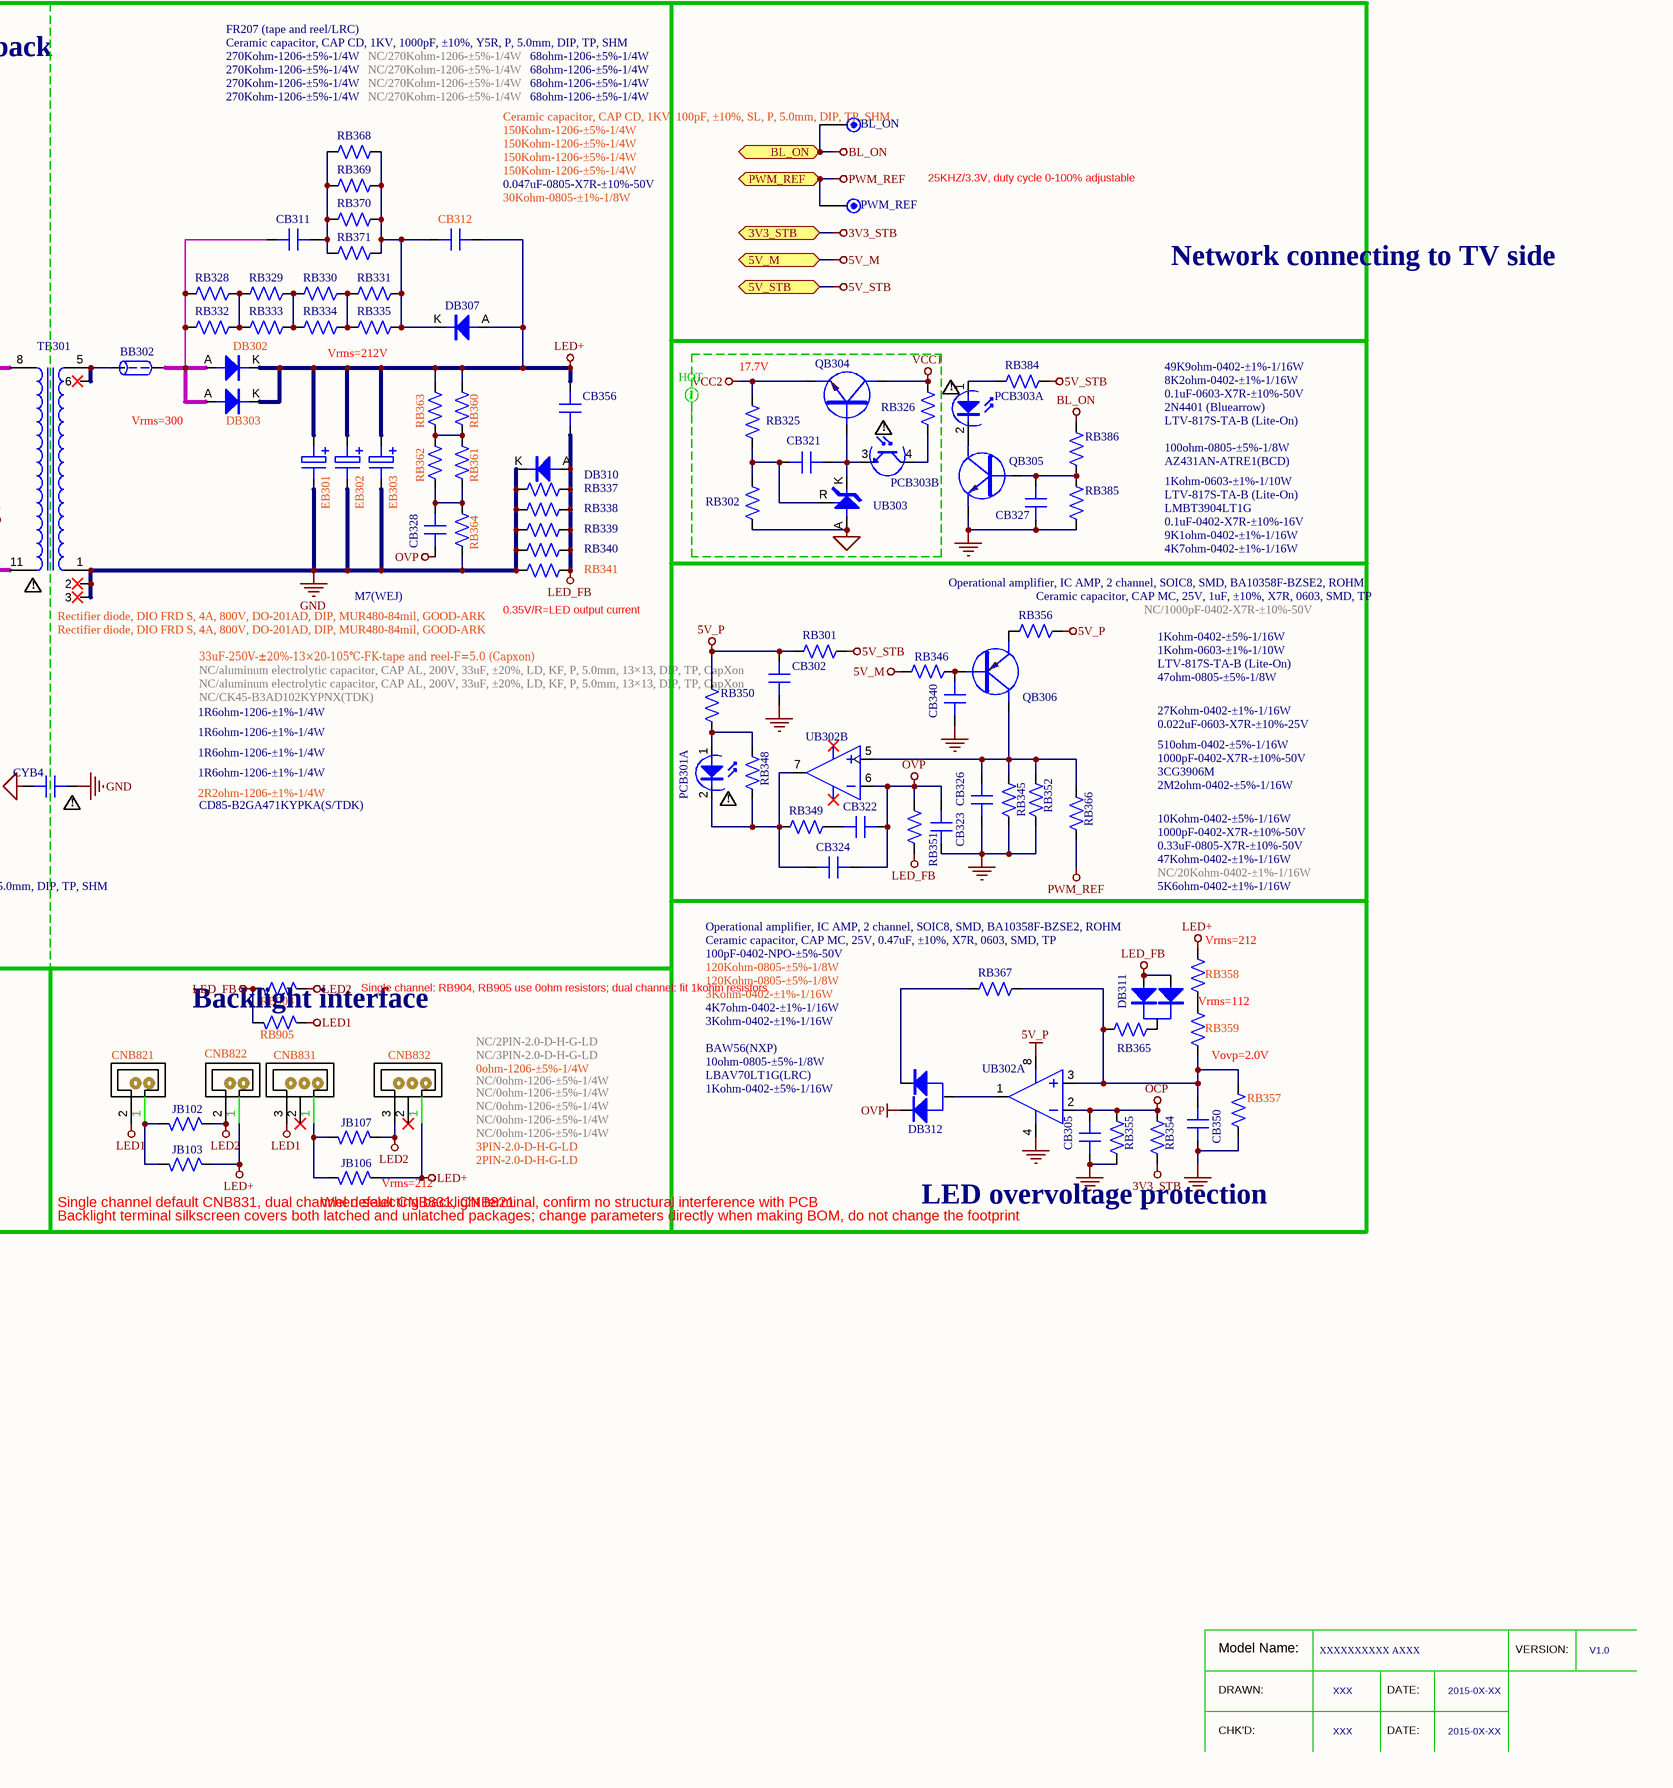
[diagram p0: PCBE84277.SchDoc, bottom right]
# Altium project MISC84277-14.PrjPCB (part 5 of 10)

## Sheet PCBE84277.SchDoc: MISC84277 (continued)

### Parts
BB101  φ3.5×6.0×0.65mm-CP (tape and reel/Xiuyida)  [LB/3.5*6*15]
BB201  φ3.5×6.0×0.65mm-CP (tape and reel/Xiuyida)  [LB/3.5*6*12.5]
BB301  φ3.5×6.0×0.65mm-CP (tape and reel/Xiuyida)  [LB/3.5*6*12.5]
BB302  φ3.5×6.0×0.65mm-CP (tape and reel/Xiuyida)  [LB/3.5*6*12.5]
BL_ON  TEST  [TP_BL]  (value not drawn)
CB2  B32672P4474K006(EPCOS)  [CAP18*7-V-15]
CB3  B32672P4474K006(EPCOS)  [CAP18*7-V-15]
CB101  100pF-0402-NPO-±5%-50V  [C0402]
CB102  0.1uF-0603-X7R-±10%-50V  [C0603]
CB103  1000pF-0402-X7R-±10%-50V  [C0402]
CB109  0.1uF-0603-X7R-±10%-50V  [C0603]
CB110  NC/1000pF-0402-X7R-±10%-50V  [C0402]
CB111  NC/1uF-0805-X7R-±10%-25V  [C0805]
CB112  NC/1uF-0805-X7R-±10%-25V  [C0805]
CB113  220PF-0805-NPO-±10%-200V  [C0805]
CB114  C242G472J20A201 (tape and reel/Faraday)  [CAP8*2.5-V-5]
CB116  Ceramic capacitor, CAP CD, 1KV, 100pF, ±10%, SL, P, 5.0mm, DIP, TP, SHM  [CAP7.5*2.5-V-5]
CB118  1000pF-0805-NPO-±10%-200V  [C0805]
CB201  0.047uF-0603-X7R-±10%-25V  [C0603]
CB204  NC/ceramic capacitor, CAP CD, 1KV, 4700pF, ±20%, Y5U, P, 5.0mm, DIP, TP, TongHao  [CAP9.8*4-V-5]
CB205  220pF-0402-NPO-±5%-50V  [C0402]
CB206  0.1uF-0603-X7R-±10%-50V  [C0603]
CB209  Ceramic capacitor, CAP CD, 1KV, 100pF, ±10%, SL, P, 5.0mm, DIP, TP, SHM  [CAP7.5*2.5-V-5]
CB211  CC45SL3AD470JYPNA(TDK)  [CAP7.5*2.5-V-5]
CB212  0.22uF-0805-X7R-±10%-50V  [C0805]
CB221  4700pF-0402-X7R-±10%-50V  [C0402]
CB301  4700pF-0402-X7R-±10%-50V  [C0402]
CB302  Ceramic capacitor, CAP MC, 25V, 1uF, ±10%, X7R, 0603, SMD, TP  [C0603]
CB303  100pF-0402-NPO-±5%-50V  [C0402]
CB304  0.1uF-0603-X7R-±10%-50V  [C0603]
CB305  100pF-0402-NPO-±5%-50V  [C0402]
CB306  C242G472J20A201 (tape and reel/Faraday)  [CAP8*2.5-V-5]
CB311  Ceramic capacitor, CAP CD, 1KV, 1000pF, ±10%, Y5R, P, 5.0mm, DIP, TP, SHM  [CAP7.5*2.5-V-5]
CB312  Ceramic capacitor, CAP CD, 1KV, 100pF, ±10%, SL, P, 5.0mm, DIP, TP, SHM  [CAP7.5*2.5-V-5]
CB316  Ceramic capacitor, CAP CD, 1KV, 100pF, ±10%, SL, P, 5.0mm, DIP, TP, SHM  [CAP7.5*2.5-V-5]
CB321  0.1uF-0603-X7R-±10%-50V  [C0603]
CB322  0.022uF-0603-X7R-±10%-25V  [C0603]
CB323  1000pF-0402-X7R-±10%-50V  [C0402]
CB324  NC/1000pF-0402-X7R-±10%-50V  [C0402]
CB326  0.33uF-0805-X7R-±10%-50V  [C0805]
CB327  0.1uF-0402-X7R-±10%-16V  [C0402]
CB328  0.047uF-0805-X7R-±10%-50V  [C0805]
CB340  1000pF-0402-X7R-±10%-50V  [C0402]
CB350  Ceramic capacitor, CAP MC, 25V, 0.47uF, ±10%, X7R, 0603, SMD, TP  [C0603]
CB356  NC/CK45-B3AD102KYPNX(TDK)  [CAP8.5*4-V-5]
CB951  NC/0.1uF-0402-X7R-±10%-16V  [C0402]
CNB1  Connect jack, 2Pin, D7.92, L, SNAP, Fool-proofing, nature, L=2.8mm, DIP, AMA  [CON2-H7.92]
CNB2  2PIN-2.0-D-H-G-LD  [SIP2/2.0D-1]
CNB812  NC/2×4PIN-2.0-L-H-F-gold plated-LK  [SIP2*4H/2.0DF-1]
CNB821  NC/2PIN-2.0-D-H-G-LD  [SIP2/2.0D-CP]
CNB822  2PIN-2.0-D-H-G-LD  [SIP2/2.0D-CP]
CNB831  NC/3PIN-2.0-D-H-G-LD  [SIP3/2.0D-CP]
CNB832  3PIN-2.0-D-H-G-LD  [SIP3/2.0D-CP]
CXB1  X capacitor, CAP X2, MP, 275VAC, 0.47uF, ±10%, S, 15mm-Mini, PC, DIP, BM  [CAP18*8.5-V-15]
CYB1  CD70-B2GA221KYPKA(S/TDK)  [CAP13*4.5-V-10]
CYB2  CD70-B2GA221KYPKA(S/TDK)  [CAP13*4.5-V-10]
CYB3  CD85-B2GA471KYPKA(S/TDK)  [CAP13*4.5-V-10]
CYB4  CD85-B2GA471KYPKA(S/TDK)  [CAP13*4.5-V-10]
DB1  1N5408G (tape and reel / GOOD-ARK)  [D3-H-20]
DB2  1N5408G (tape and reel / GOOD-ARK)  [D3-H-20]
DB3  1N5408G (tape and reel / GOOD-ARK)  [D3-H-20]
DB4  1N5408G (tape and reel / GOOD-ARK)  [D3-H-20]
DB101  MBRB10150CT(GOOD-ARK)  [D2PAK3]
DB102  LBAV70LT1G(LRC)  [SO-23]
DB105  FR107 (tape and reel/LRC)  [D1-H-12.5]
DB106  FR207 (tape and reel/LRC)  [D2-H-17.5]
DB201  Rectifier diode, DIO FRD S, 8A, 600V, ITO-220AC, DIP, UGF8J C0G, TSC  [TO-220-AK-H]
DB202  NC/GS3J-B(GULF)  [DIODE-SMB-1]
DB203  NC/GS3J-B(GULF)  [DIODE-SMB-1]
DB204  LBAV70LT1G(LRC)  [SO-23]
DB302  Rectifier diode, DIO FRD S, 4A, 800V, DO-201AD, DIP, MUR480-84mil, GOOD-ARK  [D3-H-20]
DB303  Rectifier diode, DIO FRD S, 4A, 800V, DO-201AD, DIP, MUR480-84mil, GOOD-ARK  [D3-H-20]
DB306  FR207 (tape and reel/LRC)  [D2-H-17.5]
DB307  FR207 (tape and reel/LRC)  [D2-H-17.5]
DB310  M7(WEJ)  [DIODE-S-2]
DB311  LBAV70LT1G(LRC)  [SO-23]
DB312  BAW56(NXP)  [SO-23-1]
DB370  NC/FF7  [DIODE-S-14]
DB371  NC/FF7  [DIODE-S-14]
DB901  NC/LBAV70LT1G(LRC)  [SO-23]
DB951  NC/LBAV70LT1G(LRC)  [SO-23]
EB101  470uF-25V-±20%-10×12.5-105℃-GF-tape and reel-F=5.0 (CapXon)  [EC(10*12.5)-V-5]
EB102  NC/270uF-16V-±20%-8×11.5-105℃-PS-short leads-F=3.5 (Capxon)  [EC(8*11)-V-3.5]
EB103  470uF-25V-±20%-10×12.5-105℃-GF-tape and reel-F=5.0 (CapXon)  [EC(10*12.5)-V-5]
EB106  47uF-50V-±20%-6.3×11-105℃-GH-tape and reel-F=2.5 (CapXon)  [EC(6.3*11)-V-2.5]
EB107  10uF-50V-±20%-5×11-105℃-GH-tape and reel-F=2.5 (CapXon)  [EC(5*11)-V-2.5]
EB201  100uF-450V-±20%-16×35.5-105℃-KM-bent leads (H=8.1mm) (Capxon)  [EC(16*37)-H-7.5]
EB301  33uF-250V-±20%-13×20-105℃-FK-tape and reel-F=5.0 (Capxon)  [EC(13*20)-H-5]
EB302  NC/aluminum electrolytic capacitor, CAP AL, 200V, 33uF, ±20%, LD, KF, P, 5.0mm, 13×13, DIP, TP, CapXon  [EC(13*13)-V-5]
EB303  NC/aluminum electrolytic capacitor, CAP AL, 200V, 33uF, ±20%, LD, KF, P, 5.0mm, 13×13, DIP, TP, CapXon  [EC(13*13)-V-5]
EVA1  NC/7×7×3mm-C-4305 fireproof foam-black  [EVA(7*7*3)]
EVA2  NC/7×7×3mm-C-4305 fireproof foam-black  [EVA(7*7*3)]
EVA3  NC/7×7×3mm-C-4305 fireproof foam-black  [EVA(7*7*3)]
EVA4  NC/7×7×3mm-C-4305 fireproof foam-black  [EVA(7*7*3)]
EVA5  NC/7×7×3mm-C-4305 fireproof foam-black  [EVA(7*7*3)]
EVA6  NC/7×7×3mm-C-4305 fireproof foam-black  [EVA(7*7*3)]
EVA7  NC/7×7×3mm-C-4305 fireproof foam-black  [EVA(7*7*3)]
FB1  2010T3.15A250VA1 (tape and reel/Huade)  [FUSE8.5*4-V-5]
GD1  7.00×8.35mm-nylon-white-WQM  [Fixed]
GD2  7.00×8.35mm-nylon-white-WQM  [Fixed]
GD3  7.00×8.35mm-nylon-white-WQM  [Fixed]
GD4  7.00×8.35mm-nylon-white-WQM  [Fixed]
GL1  SLD-8854W  [Silica gel-20]
GL2  SLD-8854W  [Silica gel-10]
GL3  NC/SLD-8854W  [Silica gel-10]
GL4  SLD-8854W  [Silica gel-10]
HSB2  40×25×5.0-black-with pins (thickness=1.5mm)-FR  [HS018]
HSB3  50×25×5.0-black-with pins (thickness=1.5mm)-FR  [HS033]
HSB6  NC/17.5×14.5×0.5- natural finish -Cu-MRD  [HS038]
JB102  NC/0ohm-1206-±5%-1/4W  [R1206]
JB103  NC/0ohm-1206-±5%-1/4W  [R1206]
JB106  NC/0ohm-1206-±5%-1/4W  [R1206]
JB107  NC/0ohm-1206-±5%-1/4W  [R1206]
LB1  SYDR1212-L003-EDL  [L/LC2/15*14.5-V7.5]
LB202  SYEQ2612-L250uA-SQ  [T/EQ2512*11]
LCB1  SYT10-L002-EDL  [L/LC4/13.5*10-V-7*6]
LCB2  SYT14-L003-JM  [L/LC4/T14-H-8*6]
MB1  PM3.0×8.0×5.5mm-silver-double washer  [SCREW]
MB2  PM3.0×8.0×5.5mm-silver-double washer  [SCREW]
ML1  Mylar sheet, Mylar, XXX  [Mylar]
MOVB1  TVR10561KSC3AGGW (short leads/Weiqin)  [VR(13*5)-V-7.5]
NTCB2  SCK102R55AMBY502 (short leads/Weiqin)  [NTC(10*5)-V5]
PCB101  LTV-817S-TA-B (Lite-On)  [OC4-S-1]  (parts A,B of 2)
PCB301  LTV-817S-TA-B (Lite-On)  [OC4-S-1]  (parts A,B of 2)
PCB303  LTV-817S-TA-B (Lite-On)  [OC4-S-1]  (parts A,B of 2)
PWM_REF  TEST  [TP_BL]  (value not drawn)
QB101  MOSFET, NMOS, 5A, 700V, 0.9ohm@ID=2.5A@VGS=10V, TO-252, MMD70R900PRH, MAGNACHIP  [TO-252-GDS]
QB102  3CG3906M  [SOT-23]
QB201  MDF13N50BTH(Magnachip)  [TO-220-GDS-H]
QB201和散热片之间  0.05g  [PCB_TIME]
QB301  MDF7N65BTH(Magnachip)  [TO-220-GDS-H]
QB301和散热片之间  0.05g  [PCB_TIME]
QB302  3CG3906M  [SOT-23]
QB304  2N4401 (Bluearrow)  [TO-92-EBC]
QB305  LMBT3904LT1G  [SOT-23]
QB306  3CG3906M  [SOT-23]
QB911  NC/2SD1857L-Q-T9N-B(UTC)  [TO-92-ECB]
QB921  NC/2SD1857L-Q-T9N-B(UTC)  [TO-92-ECB]
QB931  NC/2SD1857L-Q-T9N-B(UTC)  [TO-92-ECB]
QB941  NC/2SD1857L-Q-T9N-B(UTC)  [TO-92-ECB]
QB951  NC/LMBT3904LT1G  [SOT-23]
RB1  1M2ohm-1206-±5%-1/4W  [R1206]
RB2  1M2ohm-1206-±5%-1/4W  [R1206]
RB3  1M2ohm-1206-±5%-1/4W  [R1206]
RB4  1M2ohm-1206-±5%-1/4W  [R1206]
RB101  330Kohm-1206-±5%-1/4W  [R1206]
RB102  330Kohm-1206-±5%-1/4W  [R1206]
RB103  10Kohm-0402-±1%-1/16W  [R0402]
RB104  47Kohm-0402-±1%-1/16W  [R0402]
RB105  510ohm-0402-±5%-1/16W  [R0402]
RB106  68ohm-0805-±5%-1/8W  [R0805]
RB107  510ohm-0402-±5%-1/16W  [R0402]
RB108  20ohm-0805-±5%-1/8W  [R0805]
RB109  10Kohm-0402-±5%-1/16W  [R0402]
RB110  10ohm-1206-±5%-1/4W  [R1206]
RB114  10ohm-1206-±5%-1/4W  [R1206]
RB115  10ohm-1206-±5%-1/4W  [R1206]
RB116  10ohm-1206-±5%-1/4W  [R1206]
RB117  10ohm-1206-±5%-1/4W  [R1206]
RB118  10ohm-1206-±5%-1/4W  [R1206]
RB123  47ohm-1206-±5%-1/4W  [R1206]
RB124  47ohm-1206-±5%-1/4W  [R1206]
RB131  2Kohm-0603-±5%-1/10W  [R0603]
RB132  3Kohm-0402-±1%-1/16W  [R0402]
RB133  3Kohm-0402-±1%-1/16W  [R0402]
RB134  4K7ohm-0402-±1%-1/16W  [R0402]
RB135  18Kohm-0402-±1%-1/16W  [R0402]
RB141  NC/2Mohm-1206-±5%-1/4W  [R1206]
RB142  NC/2Mohm-1206-±5%-1/4W  [R1206]
RB143  NC/0ohm-0402-±5%-1/16W  [R0402]
RB144  100Kohm-1206-±5%-1/4W  [R1206]
RB145  100Kohm-1206-±5%-1/4W  [R1206]
RB146  100Kohm-1206-±5%-1/4W  [R1206]
RB147  100Kohm-1206-±5%-1/4W  [R1206]
RB148  MOF-0R27ohm-±5%-2WS (tape and reel/Futaba)  [R2-H-17.5]
RB201  1Mohm-1206-±1%-1/4W  [R1206]
RB202  1Mohm-1206-±1%-1/4W  [R1206]
RB203  1Mohm-1206-±1%-1/4W  [R1206]
RB204  1Mohm-1206-±1%-1/4W  [R1206]
RB205  560kohm-0402-±1%-1/16W  [R0402]
RB206  27Kohm-0402-±1%-1/16W  [R0402]
RB209  39Kohm-0805-±1%-1/8W  [R0805]
RB210  10ohm-1206-±5%-1/4W  [R1206]
RB212  47ohm-0805-±5%-1/8W  [R0805]
RB213  20ohm-0805-±5%-1/8W  [R0805]
RB214  10Kohm-0402-±5%-1/16W  [R0402]
RB215  510ohm-0402-±5%-1/16W  [R0402]
RB217  MOF-0R1ohm-±5%-2WS (tape and reel/Futaba)  [R2-H-17.5]
RB218  1R6ohm-1206-±1%-1/4W  [R1206]
RB219  22ohm-1206-±5%-1/4W  [R1206]
RB220  22ohm-1206-±5%-1/4W  [R1206]
RB221  1Kohm-0402-±5%-1/16W  [R0402]
RB223  22ohm-1206-±5%-1/4W  [R1206]
RB224  22ohm-1206-±5%-1/4W  [R1206]
RB225  10Kohm-0402-±5%-1/16W  [R0402]
RB226  47Kohm-0402-±1%-1/16W  [R0402]
RB227  NC/0ohm-0402-±5%-1/16W  [R0402]
RB301  47ohm-0805-±5%-1/8W  [R0805]
RB302  8K2ohm-0402-±1%-1/16W  [R0402]
RB303  NC/10Kohm-0402-±5%-1/16W  [R0402]
RB304  47Kohm-0402-±1%-1/16W  [R0402]
RB305  510ohm-0402-±5%-1/16W  [R0402]
RB306  47ohm-0805-±5%-1/8W  [R0805]
RB307  510ohm-0402-±5%-1/16W  [R0402]
RB308  20ohm-0805-±5%-1/8W  [R0805]
RB309  10Kohm-0402-±5%-1/16W  [R0402]
RB310  MOF-0R22ohm-±5%-2WS (tape and reel/Futaba)  [R2-H-17.5]
RB314  10ohm-1206-±5%-1/4W  [R1206]
RB315  10ohm-1206-±5%-1/4W  [R1206]
RB317  330Kohm-1206-±5%-1/4W  [R1206]
RB318  330Kohm-1206-±5%-1/4W  [R1206]
RB319  330Kohm-1206-±5%-1/4W  [R1206]
RB320  330Kohm-1206-±5%-1/4W  [R1206]
RB321  330Kohm-1206-±5%-1/4W  [R1206]
RB322  330Kohm-1206-±5%-1/4W  [R1206]
RB323  330Kohm-1206-±5%-1/4W  [R1206]
RB324  330Kohm-1206-±5%-1/4W  [R1206]
RB325  49K9ohm-0402-±1%-1/16W  [R0402]
RB326  100ohm-0805-±5%-1/8W  [R0805]
RB328  270Kohm-1206-±5%-1/4W  [R1206]
RB329  270Kohm-1206-±5%-1/4W  [R1206]
RB330  270Kohm-1206-±5%-1/4W  [R1206]
RB331  270Kohm-1206-±5%-1/4W  [R1206]
RB332  NC/270Kohm-1206-±5%-1/4W  [R1206]
RB333  NC/270Kohm-1206-±5%-1/4W  [R1206]
RB334  NC/270Kohm-1206-±5%-1/4W  [R1206]
RB335  NC/270Kohm-1206-±5%-1/4W  [R1206]
RB337  1R6ohm-1206-±1%-1/4W  [R1206]
RB338  1R6ohm-1206-±1%-1/4W  [R1206]
RB339  1R6ohm-1206-±1%-1/4W  [R1206]
RB340  1R6ohm-1206-±1%-1/4W  [R1206]
RB341  2R2ohm-1206-±1%-1/4W  [R1206]
RB345  5K6ohm-0402-±1%-1/16W  [R0402]
RB346  510ohm-0402-±5%-1/16W  [R0402]
RB347  NC/MOF-300Kohm-±5%-2WS (tape and reel/Futaba)  [R2-H-17.5]
RB348  1Kohm-0402-±5%-1/16W  [R0402]
RB349  27Kohm-0402-±1%-1/16W  [R0402]
RB350  1Kohm-0603-±1%-1/10W  [R0603]
RB351  10Kohm-0402-±5%-1/16W  [R0402]
RB352  NC/20Kohm-0402-±1%-1/16W  [R0402]
RB354  3Kohm-0402-±1%-1/16W  [R0402]
RB355  4K7ohm-0402-±1%-1/16W  [R0402]
RB356  2M2ohm-0402-±5%-1/16W  [R0402]
RB357  3Kohm-0402-±1%-1/16W  [R0402]
RB358  120Kohm-0805-±5%-1/8W  [R0805]
RB359  120Kohm-0805-±5%-1/8W  [R0805]
RB360  150Kohm-1206-±5%-1/4W  [R1206]
RB361  150Kohm-1206-±5%-1/4W  [R1206]
RB362  150Kohm-1206-±5%-1/4W  [R1206]
RB363  150Kohm-1206-±5%-1/4W  [R1206]
RB364  30Kohm-0805-±1%-1/8W  [R0805]
RB365  10ohm-0805-±5%-1/8W  [R0805]
RB366  47Kohm-0402-±1%-1/16W  [R0402]
RB367  1Kohm-0402-±5%-1/16W  [R0402]
RB368  68ohm-1206-±5%-1/4W  [R1206]
RB369  68ohm-1206-±5%-1/4W  [R1206]
RB370  68ohm-1206-±5%-1/4W  [R1206]
RB371  68ohm-1206-±5%-1/4W  [R1206]
RB384  1Kohm-0603-±1%-1/10W  [R0603]
RB385  4K7ohm-0402-±1%-1/16W  [R0402]
RB386  9K1ohm-0402-±1%-1/16W  [R0402]
RB391  22ohm-1206-±5%-1/4W  [R1206]
RB392  22ohm-1206-±5%-1/4W  [R1206]
RB901  NC/470ohm-1206-±5%-1/4W  [R1206]
RB902  NC/470ohm-1206-±5%-1/4W  [R1206]
RB903  NC/470ohm-1206-±5%-1/4W  [R1206]
RB904  0ohm-1206-±5%-1/4W  [R1206]
RB905  NC/0ohm-1206-±5%-1/4W  [R1206]
RB911  NC/10ohm-1206-±5%-1/4W  [R1206]
RB912  NC/10ohm-1206-±5%-1/4W  [R1206]
RB913  NC/10ohm-1206-±5%-1/4W  [R1206]
RB921  NC/10ohm-1206-±5%-1/4W  [R1206]
RB922  NC/10ohm-1206-±5%-1/4W  [R1206]
RB923  NC/10ohm-1206-±5%-1/4W  [R1206]
RB931  NC/10ohm-1206-±5%-1/4W  [R1206]
RB932  NC/10ohm-1206-±5%-1/4W  [R1206]
RB933  NC/10ohm-1206-±5%-1/4W  [R1206]
RB941  NC/10ohm-1206-±5%-1/4W  [R1206]
RB942  NC/10ohm-1206-±5%-1/4W  [R1206]
RB943  NC/10ohm-1206-±5%-1/4W  [R1206]
RB951  NC/2Kohm-0402-±1%-1/16W  [R0402]
RB952  NC/20Kohm-1206-±5%-1/4W  [R1206]
TB101  SYEQ2612-T012A-YX  [T/EQ2512*11]
TB301  SYEQ32 (large-size constant current)  [T/EQ3214*11]
TP-TDT  (no value)  [TP-TDT]
UB101  PWM controller, IC PWM Controller, 65KHZ, SOT23-6, SMD, OB2273C, ON-Bright  [SOT-26]
UB102  AZ431AN-ATRE1(BCD)  [SOT-23-RAK]
UB201  PWM controller, IC PWM Controller, 300KHz, SOP-8, SMD, FAN7930CMX_G, Fairchild  [SO-8A]
UB301  PWM controller, IC PWM Controller, 65KHZ, SOT23-6, SMD, OB2273C, ON-Bright  [SOT-26]
UB302  Operational amplifier, IC AMP, 2 channel, SOIC8, SMD, BA10358F-BZSE2, ROHM  [SO-8A]  (parts A,B of 2)
UB303  AZ431AN-ATRE1(BCD)  [SOT-23-RAK]
ZDB101  BZX84C24 (Bluearrow)  [SO-23]

### Blocks framed on the sheet
EB101 and EB102 compatible: EB101 EB102
PFC circuit: BB201 CB2 CB3 CB201 CB204-CB206 CB209 CB211 CB212 CB221 DB201-DB204 EB201 LB1 LB202 QB201 RB201-RB206 RB209 RB210 RB212-RB215 RB217-RB221 RB223-RB227 TP-TDT UB201
Accessories and structural parts, etc.: EVA1-EVA7 GD1-GD4 GL1-GL4 HSB2 HSB3 HSB6 MB1 MB2 ML1 QB201和散热片之间 QB301和散热片之间

### Ports
3V3_STB, 5V_M, 5V_STB, BL_ON, PWM_REF

### Nets
3V3_STB: RB354.2 ; port 3V3_STB
5V_M: DB901.1 DB901.3 RB346.1 ; port 5V_M
5V_P: CB302.2 RB301.1 RB350.2 RB356.2 UB302.8
5V_STB: RB301.2 RB384.1 ; port 5V_STB
12V: CNB2.2 DB101.2 EB101.1 EB102.1 EB103.1 HSB6.1 HSB6.2 RB123.2 RB124.2 RB131.1 RB135.1
380V: CB204.2 DB201.K DB203.K EB201.1 RB117.1 RB118.1 RB144.1 RB146.1 RB201.1 RB219.2 RB220.2 RB314.2 RB315.2 RB317.2 RB318.2 RB319.2 RB320.2 RB347.2 TB101.1 TB301.8 TP-TDT.1
BL_ON: BL_ON.1 RB386.2 ; port BL_ON
BRO: RB104.2 RB143.2 UB101.3(NC)
BRO1: RB304.1 UB301.3(NC)
COMP: CB301.2 PCB301.4 UB301.2(COMP)
CS: CB303.1 RB303.1 RB305.1 UB301.4(CS)
D: BB301.2 TB301.11
GND: CB302.1 CB305.2 CB323.1 CB326.2 CB327.2 CB340.2 CB350.1 CB951.2 CNB2.1 CNB812.7 CNB812.8 CYB1.1 CYB2.1 CYB3.2 CYB4.2 DB310.K EB101.2 EB102.2 EB103.2 EB301.2 EB302.2 EB303.2 QB305.E QB951.E RB134.2 RB337.1 RB338.1 RB339.1 RB340.1 RB341.1 RB345.2 RB352.2 RB355.2 RB357.1 RB364.1 RB385.1 RB951.1 TB101.8 TB101.9 TB301.1 TB301.2 TB301.3 UB102.A UB302.4
L: DB1.A DB4.K LCB2.3 RB101.1 RB141.2
L-1: CNB1.1 FB1.1
L-2: FB1.2 LCB1.2
L-3: CXB1.1 CYB1.2 LCB1.3 LCB2.2 MOVB1.2 RB1.1 RB2.1
L-N: RB1.2 RB2.2 RB3.1 RB4.1
LED1: CNB821.2 CNB831.3 DB951.3 QB911.C QB921.C RB905.1
LED2: CNB822.2 CNB832.3 DB951.1 JB102.2 JB107.1 QB931.C QB941.C RB904.1
LED+: CB312.2 CB356.2 CNB822.1 CNB832.1 DB302.K DB303.K DB307.A EB301.1 EB302.1 EB303.1 JB103.1 JB106.1 RB358.1 RB360.2 RB363.2
LED_FB: CB356.1 CNB812.5 CNB812.6 DB310.A DB311.1 DB311.3 RB337.2 RB338.2 RB339.2 RB340.2 RB341.2 RB351.1 RB904.2 RB905.2 RB911.1 RB912.1 RB913.1 RB921.1 RB922.1 RB923.1 RB931.1 RB932.1 RB933.1 RB941.1 RB942.1 RB943.1
N-1: CNB1.3 LCB1.1
N-2: CXB1.2 CYB2.2 LCB1.4 LCB2.1 MOVB1.1 RB3.2 RB4.2
N-3: DB2.A DB3.K LCB2.4
OCP: CB305.1 QB951.C RB354.1 RB355.1 UB302.2
OUT: RB306.1 RB307.1 UB301.6(GATE)
OVP: CB322.2 CB323.2 CB324.2 CB328.1 DB312.2 RB351.2 UB302.6
PFC_CS: CB205.2 RB215.1 UB201.4(CS)
PWM_REF: PWM_REF.1 RB366.2 ; port PWM_REF
SGND: CB2.2 CB3.2 CB101.2 CB102.2 CB103.2 CB111.1 CB112.1 CB201.1 CB204.1 CB205.1 CB206.1 CB212.2 CB221.1 CB301.1 CB303.2 CB304.2 CYB3.1 CYB4.1 DB3.A DB4.A DB371.K EB106.2 EB107.2 EB201.2 HSB2.3 HSB3.1 LB202.6 PCB101.3 PCB301.3 RB103.1 RB104.1 RB148.1 RB205.1 RB206.2 RB217.1 RB218.1 RB226.1 RB227.1 RB302.2 RB303.2 RB304.2 RB310.1 TB101.5 TP-TDT.2 UB101.1(GND) UB201.6(GND) UB301.1(GND) UB303.A ZDB101.1 ZDB101.3
Vbridge: CB2.1 DB202.A LB1.1 NTCB2.1
VCC1: DB105.K EB106.1 QB304.C RB110.2 RB116.1 RB326.1
VCC2: CB304.1 QB304.E RB210.2 RB325.2 UB301.5(VCC)
ZCD: LB202.5 RB209.2
H: BB101.1 CB116.2 DB106.A QB101.D
NetBB101_2: BB101.2 TB101.3
NetBB201_1: BB201.1 LB202.3
NetBB201_2: BB201.2 CB209.2 CB211.1 DB201.A QB201.D
NetBB301_1: BB301.1 CB316.2 DB306.A QB301.D
NetBB302_1: BB302.1 TB301.5 TB301.6
NetBB302_2: BB302.2 CB311.1 DB302.A DB303.A RB328.1 RB332.1
NetCB3_1: CB3.1 LB1.2 LB202.1
NetCB101_1: CB101.1 RB103.2 RB105.1 UB101.4(CS)
NetCB102_1: CB102.1 DB102.2 EB107.1 RB102.2 UB101.5(VCC)
NetCB103_1: CB103.1 PCB101.4 UB101.2(COMP)
NetCB109_1: CB109.1 CB110.1 PCB101.2 RB132.2 UB102.K
NetCB109_2: CB109.2 RB133.1
NetCB110_2: CB110.2 RB133.2 RB134.1 RB135.2 UB102.R
NetCB111_2: CB111.2 CB112.2 RB142.1 RB143.1
NetCB113_1: CB113.1 DB105.A RB114.1 RB115.1
NetCB113_2: CB113.2 RB116.2
NetCB114_1: CB114.1 RB117.2 RB118.2
NetCB114_2: CB114.2 DB106.K RB145.2 RB147.2
NetCB116_1: CB116.1 QB101.S RB105.2 RB108.2 RB109.2 RB148.2
NetCB118_1: CB118.1 DB101.1 DB101.3 TB101.10
NetCB118_2: CB118.2 RB123.1 RB124.1
NetCB201_2: CB201.2 RB225.1 UB201.3(COMP)
NetCB206_2: CB206.2 RB210.1 UB201.8(VCC)
NetCB209_1: CB209.1 RB219.1 RB220.1
NetCB211_2: CB211.2 RB223.1 RB224.1
NetCB212_1: CB212.1 RB225.2 RB227.2
NetCB221_2: CB221.2 RB221.1
NetCB306_1: CB306.1 RB314.1 RB315.1
NetCB306_2: CB306.2 DB306.K RB321.1 RB322.1 RB323.1 RB324.1 RB347.1
NetCB311_2: CB311.2 RB368.1 RB369.1 RB370.1 RB371.1
NetCB312_1: CB312.1 DB307.K RB331.2 RB335.2 RB368.2 RB369.2 RB370.2 RB371.2
NetCB316_1: CB316.1 RB391.1 RB392.1
NetCB321_1: CB321.1 PCB303.3 QB304.B UB303.K
NetCB321_2: CB321.2 RB302.1 RB325.1 UB303.R
NetCB322_1: CB322.1 RB349.2
NetCB324_1: CB324.1 PCB301.2 RB348.2 RB349.1 UB302.7
NetCB326_1: CB326.1 QB306.C RB345.1 RB352.1 RB366.1 UB302.5
NetCB327_1: CB327.1 QB305.B RB385.2 RB386.1
NetCB328_2: CB328.2 RB361.1 RB362.1 RB364.2
NetCB340_1: CB340.1 QB306.B RB346.2
NetCB350_2: CB350.2 RB357.2 RB359.2 RB365.2 RB367.2 UB302.3
NetCB951_1: CB951.1 QB951.B RB951.2 RB952.1
NetCNB821_1: CNB821.1 JB102.1 JB103.2
NetCNB831_1: CNB831.1 JB106.2 JB107.2
NetDB1_K: DB1.K DB2.K NTCB2.2
NetDB102_1: DB102.1 DB102.3 RB110.1 ZDB101.2
NetDB202_K: DB202.K DB203.A
NetDB204_1: DB204.1 DB204.3 QB201.G RB212.2 RB214.2
NetDB204_2: DB204.2 RB213.2
NetDB311_2: DB311.2 RB365.1
NetDB312_1: DB312.1 RB367.1
NetDB312_3: DB312.3 UB302.1
NetDB370_A: DB370.A QB301.S RB305.2 RB308.2 RB309.1 RB310.2 RB391.2 RB392.2
NetDB370_K: DB370.K DB371.A
NetDB901_2: DB901.2 RB901.2 RB902.2 RB903.2
NetDB951_2: DB951.2 RB952.2
NetPCB101_1: PCB101.1 RB131.2 RB132.1
NetPCB301_1: PCB301.1 RB348.1 RB350.1
NetPCB303_1: PCB303.1 RB384.2
NetPCB303_2: PCB303.2 QB305.C
NetPCB303_4: PCB303.4 RB326.2
NetQB101_G: QB101.G QB102.E RB106.2 RB109.1
NetQB102_B: QB102.B RB107.2
NetQB102_C: QB102.C RB108.1
NetQB201_S: QB201.S RB214.1 RB215.2 RB217.2 RB218.2 RB223.2 RB224.2
NetQB301_G: QB301.G QB302.E RB306.2 RB309.2
NetQB302_B: QB302.B RB307.2
NetQB302_C: QB302.C RB308.1
NetQB306_E: QB306.E RB356.1
NetQB911_B: QB911.B QB921.B QB931.B QB941.B RB901.1 RB902.1 RB903.1
NetQB911_E: QB911.E RB911.2 RB912.2 RB913.2
NetQB921_E: QB921.E RB921.2 RB922.2 RB923.2
NetQB931_E: QB931.E RB931.2 RB932.2 RB933.2
NetQB941_E: QB941.E RB941.2 RB942.2 RB943.2
NetRB101_2: RB101.2 RB102.1
NetRB106_1: RB106.1 RB107.1 UB101.6(GATE)
NetRB114_2: RB114.2 RB115.2 TB101.6
NetRB141_1: RB141.1 RB142.2
NetRB144_2: RB144.2 RB145.1 RB146.2 RB147.1
NetRB201_2: RB201.2 RB202.1
NetRB202_2: RB202.2 RB203.1
NetRB203_2: RB203.2 RB204.1
NetRB204_2: RB204.2 RB205.2 RB206.1 RB221.2 UB201.1(INV)
NetRB209_1: RB209.1 UB201.5(ZCD)
NetRB212_1: RB212.1 RB213.1 UB201.7(OUT)
NetRB226_2: RB226.2 UB201.2(RDY)
NetRB317_1: RB317.1 RB318.1 RB319.1 RB320.1 RB321.2 RB322.2 RB323.2 RB324.2
NetRB328_2: RB328.2 RB329.1 RB332.2 RB333.1
NetRB329_2: RB329.2 RB330.1 RB333.2 RB334.1
NetRB330_2: RB330.2 RB331.1 RB334.2 RB335.1
NetRB358_2: RB358.2 RB359.1
NetRB360_1: RB360.1 RB361.2 RB362.2 RB363.1

Not connected (* = marked no-connect by the designer): CNB812 1* 2* 3* 4*; CNB831 2*; CNB832 2*; HSB2 2*; MB1 1*; MB2 1*; TB101 7* 11*

### Layout directives
net class HOT: 380V, BRO, BRO1, COMP, CS, D, H, L, L-1, L-2, L-3, L-N, N-1, N-2, N-3, OUT, PFC_CS, SGND, Vbridge, VCC1, VCC2, ZCD
net class POWER: (no net found under the mark)

### Notes on the sheet
- Configuration: power 108W; constant-current voltage 111-212V
- (For other specifications, change the corresponding orange material)
- Note:
- When TB101 uses SYEQ2612-T012019,
- Sense resistor must use 0.27ohm, change RB103 to 10K
- Standby circuit
- RB337-RB344 high-voltage section uses 1R6*4, +2R2; low-voltage section uses 1R6*7
- RB360-RB364 high-voltage section uses 150K*4, +30K; low-voltage section uses 100K*4+30K
- Brown-out circuit:
- Fit when fast power-down is needed, otherwise cancel
- (near RB141) When fitted, change RB104 to 120K; chip uses 7537
- (near TB101) !
- (near RB141) AC   Vrms=264
- Vrms=380
- When making certification schematic for 12V output, change to the correct footprint
- EMI circuit
- AC   Vrms=140
- (near CB114) Vrms=300
- (near BB101) Vrms=380
- (near RB124) (Download latest library file, search SYEQ2612-T012A-JM)
- (near RB143) Place close to IC
- (near CNB1) !
- (near FB1) T3.15AL 250V~
- (near FB1) !
- (near LCB1) !
- (near CXB1) !
- (near RB1) !
- (near RB2) !
- (near LCB2) !
- AC   Vrms=264
- (near DB1) !
- (near NTCB2) !
- (near NTCB2) Vrms=380
- (near CYB1) !
- (near RB3) !
- !
- (near DB4) !
- (near DB3) !
- (near DB2) !
- (near RB4) !
- (near CYB2) !
- (near CYB3) !
- EB201 default KM, change when making BOM
- (near LB202) !
- Constant-current circuit - flyback
- Vrms=285
- Normal use [100uF-450V-±20%-16×35.5-105℃-KM-bent leads (H=8.1mm) (Capxon)]
- Vrms=190
- Vrms=95
- 25KHZ/3.3V, duty cycle 0-100% adjustable
- (near PWM_REF) Network connecting to TV side
- Vrms=212V
- 17.7V
- RB306 default 47ohm in schematic; increase if EMI fails
- Vrms=300
- (near QB304) !
- (near CB306) Vrms=300
- (near TB301) !
- 0.35V/R=LED output current
- Current sharing circuit
- (near DB951) LED protection circuit
- (near CB301) !
- (near CYB4) !
- Cancel for single-channel constant current
- Backlight interface
- Single channel: RB904, RB905 use 0ohm resistors; dual channel: fit 1kohm resistors
- Vrms=112
- (near RB358) Vrms=212
- (near RB359) Vovp=2.0V
- Reserved fireproof foam position must meet both half-wrap and full-wrap requirements; update BOM when selecting
- EB201 bottom
- (near HSB6) !
- (near HSB2) !
- (near HSB2) HSB1  FOR QB201
- (near HSB3) !
- (near HSB3) HSB3  FOR QB301
- (near JB106) Single channel default CNB831, dual channel default CNB831, CNB821
- (near JB106) When selecting backlight terminal, confirm no structural interference with PCB
- (near JB106) Vrms=212
- LED overvoltage protection
- EB301 bottom
- LB2 bottom
- DB201 bottom
- Backlight terminal silkscreen covers both latched and unlatched packages; change parameters directly when making BOM, do not change the footprint
- (near QB301和散热片之间) Note: adjust accessories and process per BOM requirements
- Lying flat
- Process
- EB201,EB301(MI),DB201
- Ref. designator
- Accessories and special process not shown in schematic
- Raised height
- XXX
- DB1,DB2,DB3,DB4,DB302,DB303
- Model Name:
- XXXXXXXXXX AXXX
- VERSION:
- V1.0
- CHK'D:
- DRAWN:
- DATE:
- 2015-0X-XX
- Title
- Size:
- Date:
- A4
- Number:
- Time:
- Revision:
- Sheet
- of
- File: